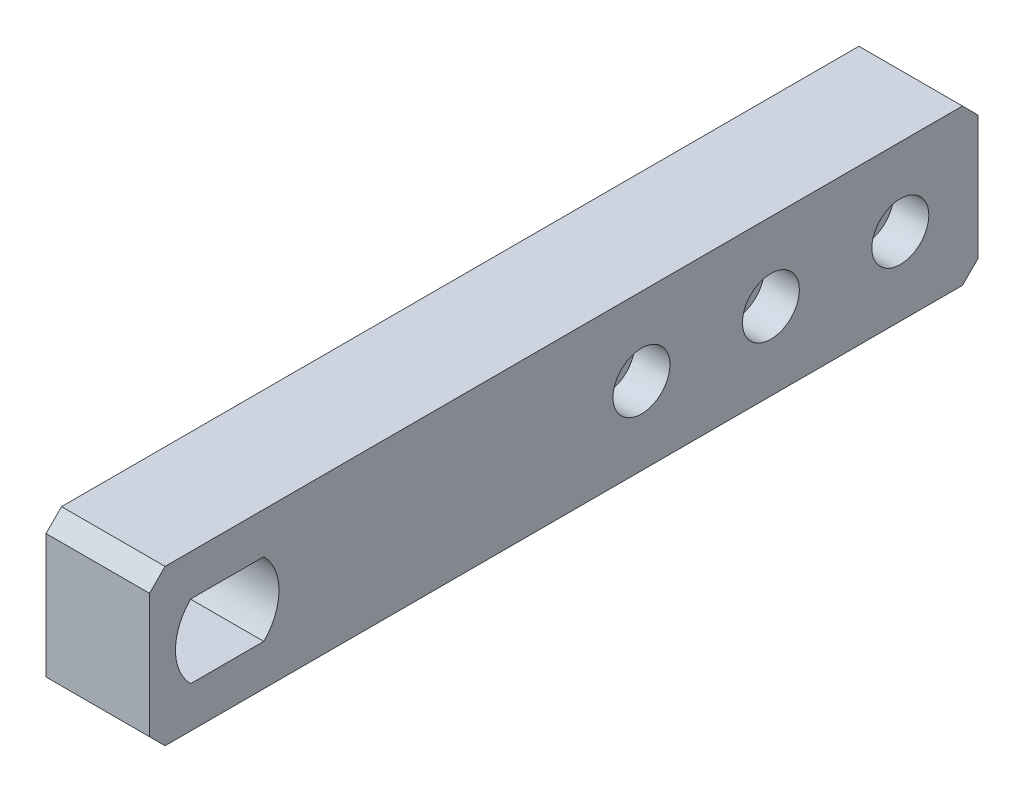
SolidWorks part; units mm, degrees
ref_plane "前视基准面" through (0, 0, 0) normal (0, 0, 1) x (1, 0, 0)
ref_plane "上视基准面" through (0, 0, 0) normal (0, 1, 0) x (1, 0, 0)
ref_plane "右视基准面" through (0, 0, 0) normal (1, 0, 0) x (0, 0, -1)
sketch "草图1" plane through (0, 0, 0) normal (1, 0, 0) x (0, 0, -1)
  line L1 (-80, 15) -> (80, 15)
  line L2 (-80, 15) -> (-80, -15)
  line L3 (-80, -15) -> (80, -15)
  line L4 (80, 15) -> (80, -15)
  line L5 (-80, 15) -> (80, -15) construction
  line L6 (-80, -15) -> (80, 15) construction
  point P0 (0, 0)
  dimension "D1" = 30
  dimension "D2" = 160
extrude "凸台-拉伸1" add sketch "草图1" along normal blind 20
sketch "草图2" plane through (20, 0, 0) normal (1, 0, 0) x (0, 0, -1)
  line L0 (-80, 15) -> (-80, -15) construction
  line L2 (-72.0622, 7.0799) -> (-57.9378, 7.0799)
  line L4 (-72.0622, -7.0799) -> (-57.9378, -7.0799)
  line L6 (-71.6036, 7.5095) -> (-58.3964, -7.5095) construction
  line L7 (-73.9504, -4.4599) -> (-56.0496, 4.4599) construction
  arc A0 (-72.0622, 7.0799) -> (-72.0622, -7.0799) centre (-65, 0) ccw
  arc A1 (-57.9378, -7.0799) -> (-57.9378, 7.0799) centre (-65, 0) ccw
  dimension "D1" = 20
  dimension "D2" = 15
extrude "切除-拉伸1" cut sketch "草图2" against normal through all
hole_wizard "打孔尺寸(%根据)内六角圆柱头螺钉的类型1" positions "草图3" profile "草图4" counterbore size "M6" standard "GB"
sketch "草图3" plane through (20, 0, 0) normal (1, 0, 0) x (0, 0, -1)
  line L0 (80, 0) -> (20.3903, 0) construction
  line L1 (80, -15) -> (80, 15) construction
  point P0 (15, 0)
  point P2 (40, 0)
  point P4 (65, 0)
  dimension "D1" = 15
  dimension "D2" = 25
  dimension "D3" = 25
sketch "草图4" plane through (20, 0, -15) normal (0, 1, 0) x (0, 0, -1)
  line L0 (0, 0) -> (0, 39.9828)
  line L1 (0, 39.9828) -> (3.3, 38)
  line L2 (3.3, 38) -> (3.3, 6.8)
  line L3 (3.3, 6.8) -> (5.5, 6.8)
  line L4 (5.5, 6.8) -> (5.5, 0)
  line L5 (5.5, 0) -> (0, 0)
  line L10 (0, 39.9828) -> (-3.3, 38) construction
  line L11 (0, -6.35) -> (0, 107.95) construction
  dimension "孔直径" = 6.6
  dimension "孔深度" = 38
  dimension "柱形沉头孔直径" = 11
  dimension "柱形沉头孔深度" = 6.8
  dimension "导头角度" = 118
chamfer "倒角1" distance 3 angle 45 4 edges at (10, 15, 80) (10, -15, 80) (10, 15, -80) (10, -15, -80)
